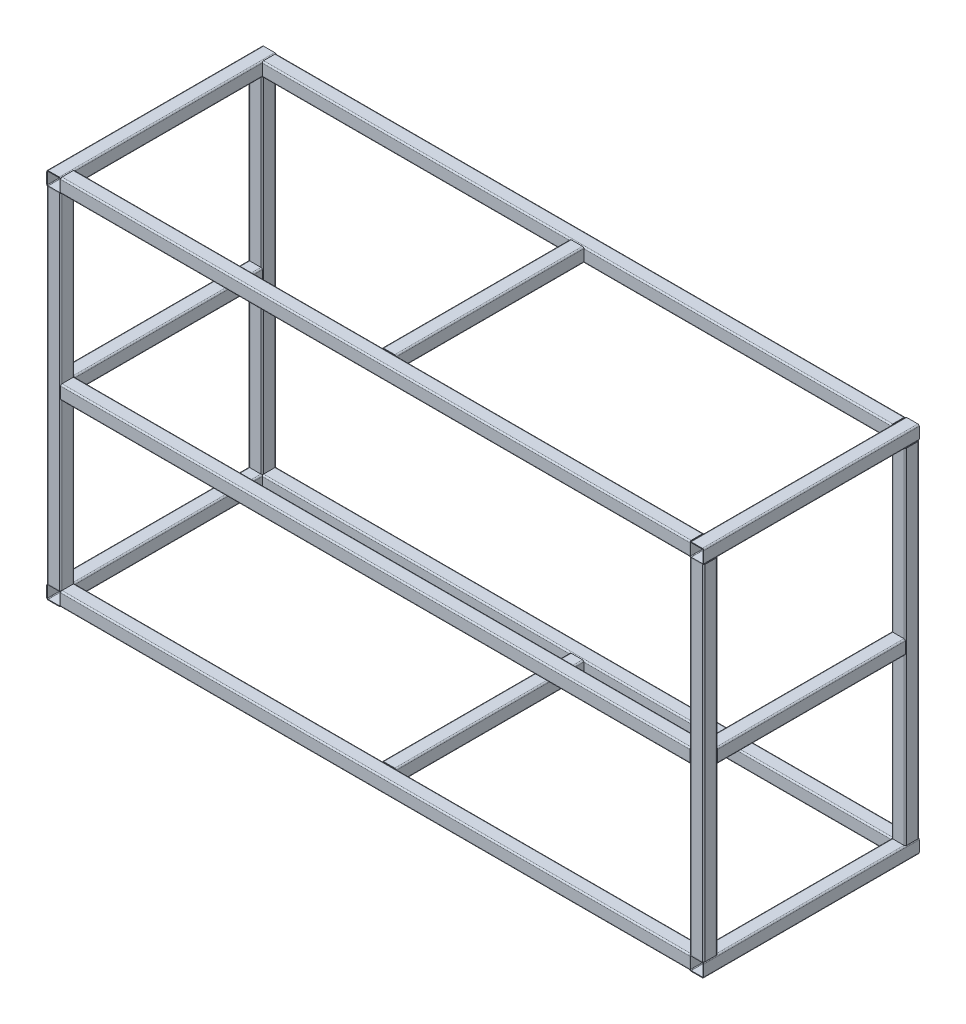
SolidWorks part; units mm, degrees
ref_plane "前视基准面" through (0, 0, 0) normal (0, 0, 1) x (1, 0, 0)
ref_plane "上视基准面" through (0, 0, 0) normal (0, 1, 0) x (1, 0, 0)
ref_plane "右视基准面" through (0, 0, 0) normal (1, 0, 0) x (0, 0, -1)
sketch "草图1" plane through (0, 0, 0) normal (0, 0, 1) x (1, 0, 0)
  line L1 (-925, -515) -> (925, -515)
  line L2 (-925, -515) -> (-925, 515)
  line L3 (-925, 515) -> (925, 515)
  line L4 (925, -515) -> (925, 515)
  line L5 (-925, -515) -> (925, 515) construction
  line L6 (-925, 515) -> (925, -515) construction
  point P0 (0, 0)
  dimension "D1" = 1030
  dimension "D2" = 1850
ref_plane "基准面1" through (0, 0, -580) normal (0, 0, 1) x (1, 0, 0)
sketch "草图2" plane through (0, 0, -580) normal (0, 0, 1) x (1, 0, 0)
  line L0 (-925, -515) -> (925, -515) construction
  line L1 (925, -515) -> (925, 515) construction
  line L2 (-925, 515) -> (925, 515) construction
  line L3 (-925, -515) -> (-925, 515) construction
  line L4 (-925, -515) -> (925, -515)
  line L5 (925, -515) -> (925, 515)
  line L6 (-925, 515) -> (925, 515)
  line L7 (-925, -515) -> (-925, 515)
sketch3d "3D草图1"
  line L0 (-925, -515, 0) -> (-925, -515, -580)
  line L1 (925, -515, 0) -> (925, -515, -580)
  line L2 (-925, 515, 0) -> (-925, 515, -580)
  line L3 (925, 515, 0) -> (925, 515, -580)
  line L4 (925, -515, -280) -> (925, 515, -280)
  dimension "D1" = 300
other "Square tube - configured 40 X 40 X 4(1)"
ref_plane "基准面2" through (-925, 515, 0) normal (1, 0, 0) x (0, 1, 0)
sketch "Sketch1" plane through (-925, 515, 0) normal (1, 0, 0) x (0, 1, 0)
  line L0 (-16, -18) -> (16, -18)
  line L1 (-18, -16) -> (-18, 16)
  line L2 (16, 18) -> (-16, 18)
  line L3 (18, 16) -> (18, -16)
  line L4 (-16, -20) -> (16, -20)
  line L5 (-20, -16) -> (-20, 16)
  line L6 (16, 20) -> (-16, 20)
  line L7 (20, 16) -> (20, -16)
  arc A0 (20, 16) -> (16, 20) centre (16, 16) ccw
  arc A1 (16, -20) -> (20, -16) centre (16, -16) ccw
  arc A2 (-20, -16) -> (-16, -20) centre (-16, -16) ccw
  arc A3 (-16, 20) -> (-20, 16) centre (-16, 16) ccw
  arc A4 (-16, 18) -> (-18, 16) centre (-16, 16) ccw
  arc A5 (18, 16) -> (16, 18) centre (16, 16) ccw
  arc A6 (16, -18) -> (18, -16) centre (16, -16) ccw
  arc A7 (-18, -16) -> (-16, -18) centre (-16, -16) ccw
  point P0 (-20, 0)
  point P1 (20, 0)
  point P2 (0, 20)
  point P3 (0, -20)
  point P4 (0, 0)
  point P5 (-20, -20)
  point P6 (20, -20)
  point P7 (20, 20)
  point P8 (-20, 20)
  point P33 (0, 0)
  dimension "D1" = 4
  dimension "Thickness" = 2
  dimension "V_leg" = 40
other "Square tube - configured 40 X 40 X 4(2)"
ref_plane "基准面3" through (925, -515, -580) normal (0, 1, 0) x (-1, 0, 0)
sketch "Sketch11" plane through (925, -515, -580) normal (0, 1, 0) x (-1, 0, 0)
  line L0 (-16, -18) -> (16, -18)
  line L1 (-18, -16) -> (-18, 16)
  line L2 (16, 18) -> (-16, 18)
  line L3 (18, 16) -> (18, -16)
  line L4 (-16, -20) -> (16, -20)
  line L5 (-20, -16) -> (-20, 16)
  line L6 (16, 20) -> (-16, 20)
  line L7 (20, 16) -> (20, -16)
  arc A0 (20, 16) -> (16, 20) centre (16, 16) ccw
  arc A1 (16, -20) -> (20, -16) centre (16, -16) ccw
  arc A2 (-20, -16) -> (-16, -20) centre (-16, -16) ccw
  arc A3 (-16, 20) -> (-20, 16) centre (-16, 16) ccw
  arc A4 (-16, 18) -> (-18, 16) centre (-16, 16) ccw
  arc A5 (18, 16) -> (16, 18) centre (16, 16) ccw
  arc A6 (16, -18) -> (18, -16) centre (16, -16) ccw
  arc A7 (-18, -16) -> (-16, -18) centre (-16, -16) ccw
  point P0 (-20, 0)
  point P1 (20, 0)
  point P2 (0, 20)
  point P3 (0, -20)
  point P4 (0, 0)
  point P5 (-20, -20)
  point P6 (20, -20)
  point P7 (20, 20)
  point P8 (-20, 20)
  point P33 (0, 0)
  dimension "D1" = 4
  dimension "Thickness" = 2
  dimension "V_leg" = 40
other "Square tube - configured 40 X 40 X 4(4)"
ref_plane "基准面4" through (-925, -515, 0) normal (0, 0, -1) x (1, 0, 0)
sketch "Sketch12" plane through (-925, -515, 0) normal (0, 0, -1) x (1, 0, 0)
  line L0 (-16, -18) -> (16, -18)
  line L1 (-18, -16) -> (-18, 16)
  line L2 (16, 18) -> (-16, 18)
  line L3 (18, 16) -> (18, -16)
  line L4 (-16, -20) -> (16, -20)
  line L5 (-20, -16) -> (-20, 16)
  line L6 (16, 20) -> (-16, 20)
  line L7 (20, 16) -> (20, -16)
  arc A0 (20, 16) -> (16, 20) centre (16, 16) ccw
  arc A1 (16, -20) -> (20, -16) centre (16, -16) ccw
  arc A2 (-20, -16) -> (-16, -20) centre (-16, -16) ccw
  arc A3 (-16, 20) -> (-20, 16) centre (-16, 16) ccw
  arc A4 (-16, 18) -> (-18, 16) centre (-16, 16) ccw
  arc A5 (18, 16) -> (16, 18) centre (16, 16) ccw
  arc A6 (16, -18) -> (18, -16) centre (16, -16) ccw
  arc A7 (-18, -16) -> (-16, -18) centre (-16, -16) ccw
  point P0 (-20, 0)
  point P1 (20, 0)
  point P2 (0, 20)
  point P3 (0, -20)
  point P4 (0, 0)
  point P5 (-20, -20)
  point P6 (20, -20)
  point P7 (20, 20)
  point P8 (-20, 20)
  point P33 (0, 0)
  dimension "D1" = 4
  dimension "Thickness" = 2
  dimension "V_leg" = 40
other "剪裁/延伸1"
other "剪裁/延伸5"
other "剪裁/延伸6"
other "剪裁/延伸17"
other "剪裁/延伸18"
other "剪裁/延伸19"
other "剪裁/延伸20"
other "剪裁/延伸21"
other "剪裁/延伸22"
other "剪裁/延伸23"
other "剪裁/延伸24"
other "剪裁/延伸25"
sketch3d "3D草图2"
  line L0 (0, -515, -580) -> (0, -515, 0)
  line L1 (-925, -515, -580) -> (925, -515, -580) construction
  line L2 (-925, -515, 0) -> (925, -515, 0) construction
  line L3 (0, 515, -580) -> (0, 515, 0)
  line L4 (-925, 515, -580) -> (925, 515, -580) construction
  line L5 (-925, 515, 0) -> (925, 515, 0) construction
  line L6 (-925, 0, -580) -> (-925, 0, 0)
  line L7 (-925, -515, -580) -> (-925, 515, -580) construction
  line L8 (-925, -515, 0) -> (-925, 515, 0) construction
  line L9 (925, 0, -580) -> (925, 0, 0)
  line L10 (925, -515, -580) -> (925, 515, -580) construction
  line L11 (925, -515, 0) -> (925, 515, 0) construction
  line L12 (925, 0, -580) -> (-925, 0, -580)
other "Square tube - configured 40 X 40 X 4(5)"
ref_plane "基准面6" through (0, -515, -580) normal (0, 0, 1) x (1, 0, 0)
sketch "Sketch14" plane through (0, -515, -580) normal (0, 0, 1) x (1, 0, 0)
  line L0 (-16, -18) -> (16, -18)
  line L1 (-18, -16) -> (-18, 16)
  line L2 (16, 18) -> (-16, 18)
  line L3 (18, 16) -> (18, -16)
  line L4 (-16, -20) -> (16, -20)
  line L5 (-20, -16) -> (-20, 16)
  line L6 (16, 20) -> (-16, 20)
  line L7 (20, 16) -> (20, -16)
  arc A0 (20, 16) -> (16, 20) centre (16, 16) ccw
  arc A1 (16, -20) -> (20, -16) centre (16, -16) ccw
  arc A2 (-20, -16) -> (-16, -20) centre (-16, -16) ccw
  arc A3 (-16, 20) -> (-20, 16) centre (-16, 16) ccw
  arc A4 (-16, 18) -> (-18, 16) centre (-16, 16) ccw
  arc A5 (18, 16) -> (16, 18) centre (16, 16) ccw
  arc A6 (16, -18) -> (18, -16) centre (16, -16) ccw
  arc A7 (-18, -16) -> (-16, -18) centre (-16, -16) ccw
  point P0 (-20, 0)
  point P1 (20, 0)
  point P2 (0, 20)
  point P3 (0, -20)
  point P4 (0, 0)
  point P5 (-20, -20)
  point P6 (20, -20)
  point P7 (20, 20)
  point P8 (-20, 20)
  point P33 (0, 0)
  dimension "D1" = 4
  dimension "Thickness" = 2
  dimension "V_leg" = 40
sketch3d "3D草图3"
  line L0 (925, 0, 0) -> (-925, 0, 0)
  line L1 (925, -515, 0) -> (925, 515, 0) construction
  line L2 (-925, -515, 0) -> (-925, 515, 0) construction
other "Square tube - configured 40 X 40 X 4(2)"
ref_plane "基准面7" through (925, 0, 0) normal (-1, 0, 0) x (0, 0, 1)
sketch "Sketch15" plane through (925, 0, 0) normal (-1, 0, 0) x (0, 0, 1)
  line L0 (-16, -18) -> (16, -18)
  line L1 (-18, -16) -> (-18, 16)
  line L2 (16, 18) -> (-16, 18)
  line L3 (18, 16) -> (18, -16)
  line L4 (-16, -20) -> (16, -20)
  line L5 (-20, -16) -> (-20, 16)
  line L6 (16, 20) -> (-16, 20)
  line L7 (20, 16) -> (20, -16)
  arc A0 (20, 16) -> (16, 20) centre (16, 16) ccw
  arc A1 (16, -20) -> (20, -16) centre (16, -16) ccw
  arc A2 (-20, -16) -> (-16, -20) centre (-16, -16) ccw
  arc A3 (-16, 20) -> (-20, 16) centre (-16, 16) ccw
  arc A4 (-16, 18) -> (-18, 16) centre (-16, 16) ccw
  arc A5 (18, 16) -> (16, 18) centre (16, 16) ccw
  arc A6 (16, -18) -> (18, -16) centre (16, -16) ccw
  arc A7 (-18, -16) -> (-16, -18) centre (-16, -16) ccw
  point P0 (-20, 0)
  point P1 (20, 0)
  point P2 (0, 20)
  point P3 (0, -20)
  point P4 (0, 0)
  point P5 (-20, -20)
  point P6 (20, -20)
  point P7 (20, 20)
  point P8 (-20, 20)
  point P33 (0, 0)
  dimension "D1" = 4
  dimension "Thickness" = 2
  dimension "V_leg" = 40
other "剪裁/延伸26"
other "剪裁/延伸27"
other "剪裁/延伸28"
other "剪裁/延伸29"
other "剪裁/延伸30"
other "剪裁/延伸31"
other "剪裁/延伸32"
other "剪裁/延伸33"
other "剪裁/延伸34"
other "剪裁/延伸35"
